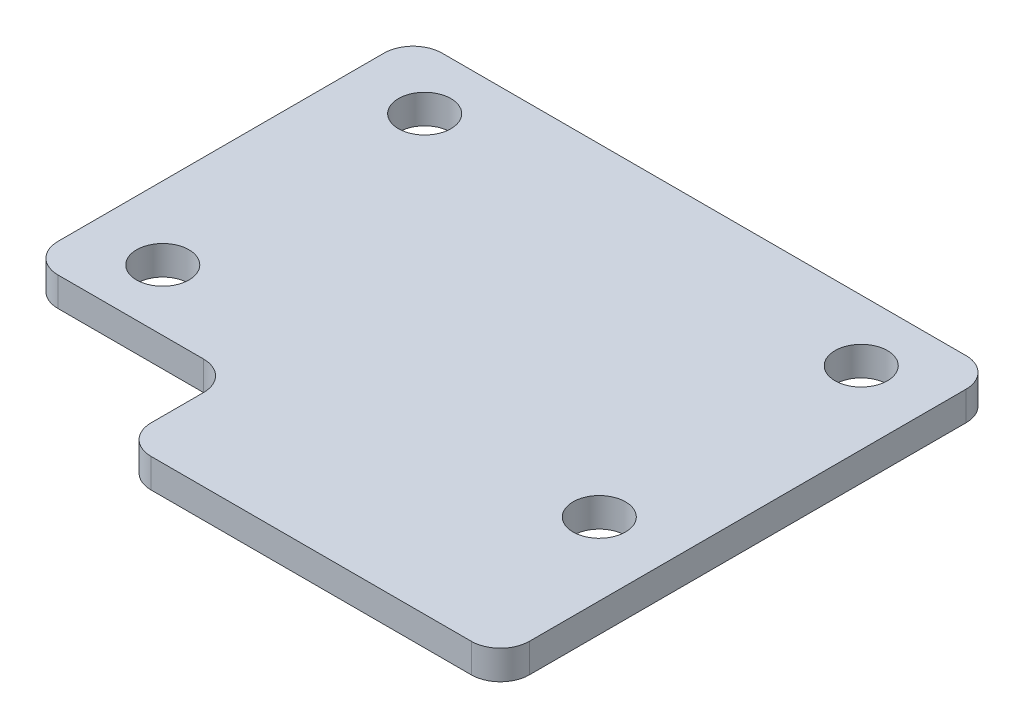
from build123d import *

# Parameters (mm, degrees)
SKETCH2_W            = 100
SKETCH2_H            = 85
BOSS_EXTRUDE1_DEPTH  = 5
M8_CLEARANCE_HOLE1_D = 9
FILLET1_R            = 5
SKETCH7_W            = 35
SKETCH7_H            = 19
CUT_EXTRUDE1_DEPTH   = 5
FILLET2_R            = 5


with BuildPart() as part:
    # Sketch2 → Boss-Extrude1 (new body)
    with BuildSketch(Plane(origin=(0, 0, 0), x_dir=(1, 0, 0), z_dir=(0, 1, 0))):
        Rectangle(SKETCH2_W, SKETCH2_H)
    extrude(amount=BOSS_EXTRUDE1_DEPTH)

    # M8 Clearance Hole1 (through all)
    with Locations(Plane(origin=(0, 5, 0), x_dir=(1, 0, 0), z_dir=(0, 1, 0))):
        with Locations((-37.5, 32), (37.5, 32), (37.5, -13), (-37.5, -13)):
            Hole(M8_CLEARANCE_HOLE1_D / 2)

    # Fillet1
    fillet1_edges = [part.edges().sort_by_distance(p)[0] for p in [
        (50, 2.5, 42.5),
        (-50, 2.5, -42.5),
        (50, 2.5, -42.5),
    ]]
    fillet(fillet1_edges, radius=FILLET1_R)

    # Sketch7 → Cut-Extrude1 (cut)
    with BuildSketch(Plane(origin=(0, 5, 0), x_dir=(1, 0, 0), z_dir=(0, 1, 0))):
        with Locations((-32.5, -33)):
            Rectangle(SKETCH7_W, SKETCH7_H)
    extrude(amount=-CUT_EXTRUDE1_DEPTH, mode=Mode.SUBTRACT)

    # Fillet2
    fillet2_edges = [part.edges().sort_by_distance(p)[0] for p in [
        (-50, 2.5, 23.5),
        (-15, 2.5, 23.5),
        (-15, 2.5, 42.5),
    ]]
    fillet(fillet2_edges, radius=FILLET2_R)


solid = part.part
